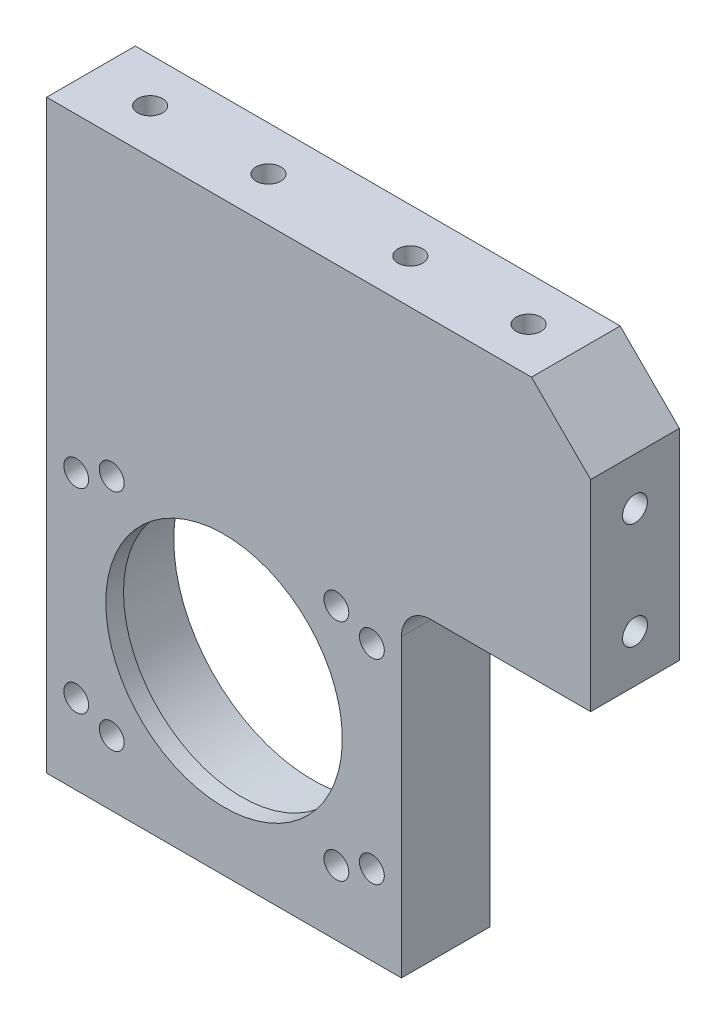
from build123d import *

# Parameters (mm, degrees)
SKETCH_1_W             = 110
SKETCH_1_H             = 100
EXTRUDE_1_DEPTH        = 7.5
SKETCH_10_R            = 23.5
CUT_EXTRUDE_1_DEPTH    = 12
SKETCH_12_R            = 20
CUT_EXTRUDE_2_DEPTH    = 76.292761936
SKETCH_13_W            = 50
SKETCH_13_H            = 55
CUT_EXTRUDE_3_DEPTH    = 76.828754441
FILLET_1_R             = 5
HOLE_WIZARD_M5_1_D     = 4.2
HOLE_WIZARD_M5_2_D     = 4.2
MOVE_FACE_1_BY         = 1
MOVE_FACE_2_BY         = 18
HOLE_WIZARD_M5_3_D     = 4.2
HOLE_WIZARD_M5_3_DEPTH = 12.4
HOLE_WIZARD_M5_3_TIP   = 1.2618073
HOLE_WIZARD_M5_4_D     = 4.2
HOLE_WIZARD_M5_4_DEPTH = 12.4
HOLE_WIZARD_M5_4_TIP   = 1.2618073
CHAMFER_2_SIZE         = 10


with BuildPart() as part:
    # 草图1 → 凸台-拉伸1 (new, symmetric)
    with BuildSketch(Plane.XY):
        Rectangle(SKETCH_1_W, SKETCH_1_H)
    extrude(amount=EXTRUDE_1_DEPTH, both=True)

    # 草图10 → 切除-拉伸1 (cut)
    with BuildSketch(Plane.XY.offset(-7.5)):
        with Locations((-25, -20)):
            Circle(SKETCH_10_R)
    extrude(amount=CUT_EXTRUDE_1_DEPTH, mode=Mode.SUBTRACT)

    # 草图12 → 切除-拉伸2 (cut, through all)
    with BuildSketch(Plane(origin=(0, 0, 4.5), x_dir=(-1, 0, 0), z_dir=(0, 0, -1))):
        with Locations((25, -20)):
            Circle(SKETCH_12_R)
    extrude(amount=-CUT_EXTRUDE_2_DEPTH, mode=Mode.SUBTRACT)

    # 草图13 → 切除-拉伸3 (cut, through all)
    with BuildSketch(Plane.XY.offset(7.5)):
        with Locations((30, -22.5)):
            Rectangle(SKETCH_13_W, SKETCH_13_H)
    extrude(amount=-CUT_EXTRUDE_3_DEPTH, mode=Mode.SUBTRACT)

    # 圆角1
    fillet_1_edges = [part.edges().sort_by_distance(p)[0] for p in [
        (5, 5, 0),
    ]]
    fillet(fillet_1_edges, radius=FILLET_1_R)

    # M5 螺纹孔1 (through all)
    with Locations(Plane(origin=(0, 0, -7.5), x_dir=(-1, 0, 0), z_dir=(0, 0, -1))):
        with Locations((0, -3.5), (0, -36.5), (50, -36.5), (50, -3.5)):
            Hole(HOLE_WIZARD_M5_1_D / 2)

    # M5 螺纹孔2 (through all)
    with Locations(Plane.XY.offset(7.5)):
        with Locations((-44, -1), (-44, -39), (-6, -39), (-6, -1)):
            Hole(HOLE_WIZARD_M5_2_D / 2)

    # Move Face 1: a face moved inward by 1.0
    extrude(part.faces().sort_by_distance((0, 50, 0))[0], amount=MOVE_FACE_1_BY, dir=(0, -1, 0), mode=Mode.SUBTRACT)

    # Move Face 2: a face moved inward by 18.0
    extrude(part.faces().sort_by_distance((55, 27, 0))[0], amount=MOVE_FACE_2_BY, dir=(-1, 0, 0), mode=Mode.SUBTRACT)

    # M5 螺纹孔3
    with Locations(Plane(origin=(0, 49, 0), x_dir=(1, 0, 0), z_dir=(0, 1, 0))):
        with Locations((19, 0), (-1, 0), (-25, 0), (-45, 0)):
            Hole(HOLE_WIZARD_M5_3_D / 2, depth=HOLE_WIZARD_M5_3_DEPTH)
            with Locations((0, 0, -(HOLE_WIZARD_M5_3_DEPTH + HOLE_WIZARD_M5_3_TIP / 2))):  # 118° drill point
                Cone(0, HOLE_WIZARD_M5_3_D / 2, HOLE_WIZARD_M5_3_TIP, mode=Mode.SUBTRACT)

    # M5 螺纹孔4
    with Locations(Plane(origin=(37, 0, 0), x_dir=(0, 0, -1), z_dir=(1, 0, 0))):
        with Locations((0, 13), (0, 31)):
            Hole(HOLE_WIZARD_M5_4_D / 2, depth=HOLE_WIZARD_M5_4_DEPTH)
            with Locations((0, 0, -(HOLE_WIZARD_M5_4_DEPTH + HOLE_WIZARD_M5_4_TIP / 2))):  # 118° drill point
                Cone(0, HOLE_WIZARD_M5_4_D / 2, HOLE_WIZARD_M5_4_TIP, mode=Mode.SUBTRACT)

    # 倒角2
    chamfer_2_edges = [part.edges().sort_by_distance(p)[0] for p in [
        (37, 49, 0),
    ]]
    chamfer(chamfer_2_edges, length=CHAMFER_2_SIZE)


solid = part.part
